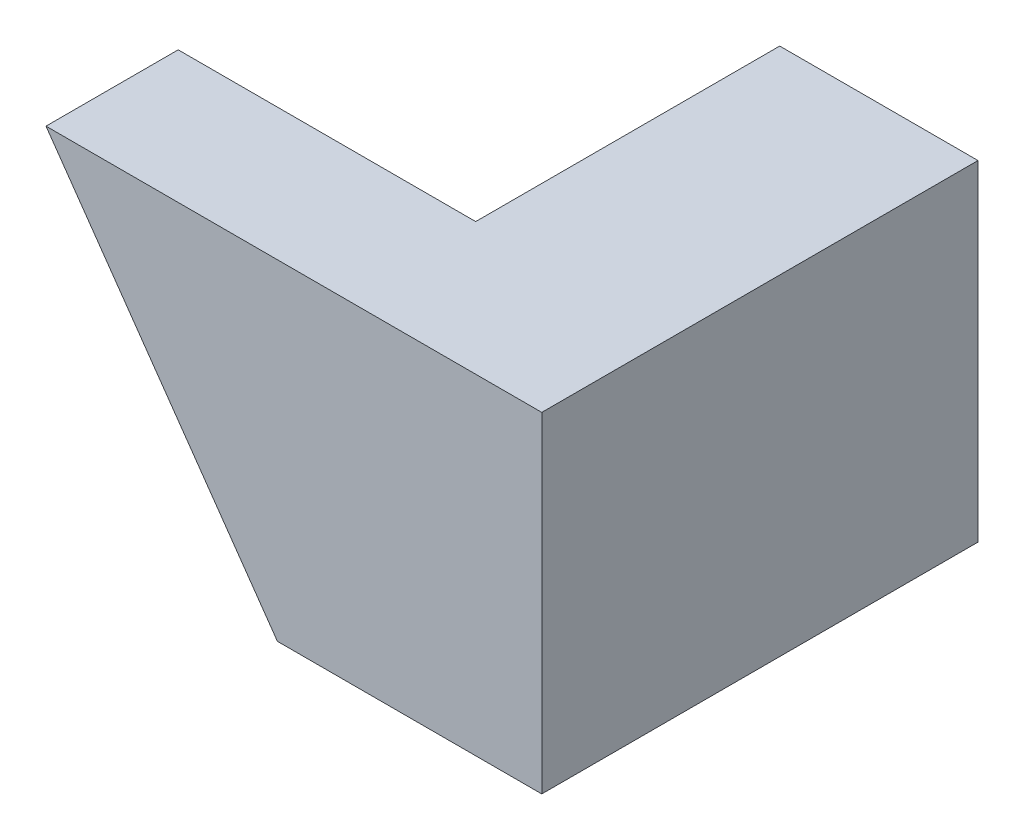
SolidWorks part; units mm, degrees
ref_plane "Front Plane" through (0, 0, 0) normal (0, 0, 1) x (1, 0, 0)
ref_plane "Top Plane" through (0, 0, 0) normal (0, 1, 0) x (1, 0, 0)
ref_plane "Right Plane" through (0, 0, 0) normal (1, 0, 0) x (0, 0, -1)
other "Configuration Table"
sketch "Sketch1" plane through (0, 0, 0) normal (0, 0, 1) x (1, 0, 0)
  line L0 (0, 0) -> (-1.7505, 2.5)
  line L1 (-1.7505, 2.5) -> (2, 2.5)
  line L2 (2, 2.5) -> (2, 0)
  line L3 (2, 0) -> (0, 0)
  dimension "D1" = 2.5
  dimension "D2" = 35
  dimension "D3" = 2
extrude "Boss-Extrude1" add sketch "Sketch1" along normal blind 1
sketch "Sketch2" plane through (0, 0, 1) normal (0, 0, 1) x (1, 0, 0)
  line L0 (2, 2.5) -> (-1.7505, 2.5) construction
  line L1 (2, 2.5) -> (0.5, 2.5)
  line L2 (2, 2.5) -> (2, 0)
  line L3 (2, 0) -> (0.5, 0)
  line L4 (0.5, 2.5) -> (0.5, 0)
  dimension "D1" = 1.5
extrude "Boss-Extrude2" add sketch "Sketch2" against normal blind 3.3
